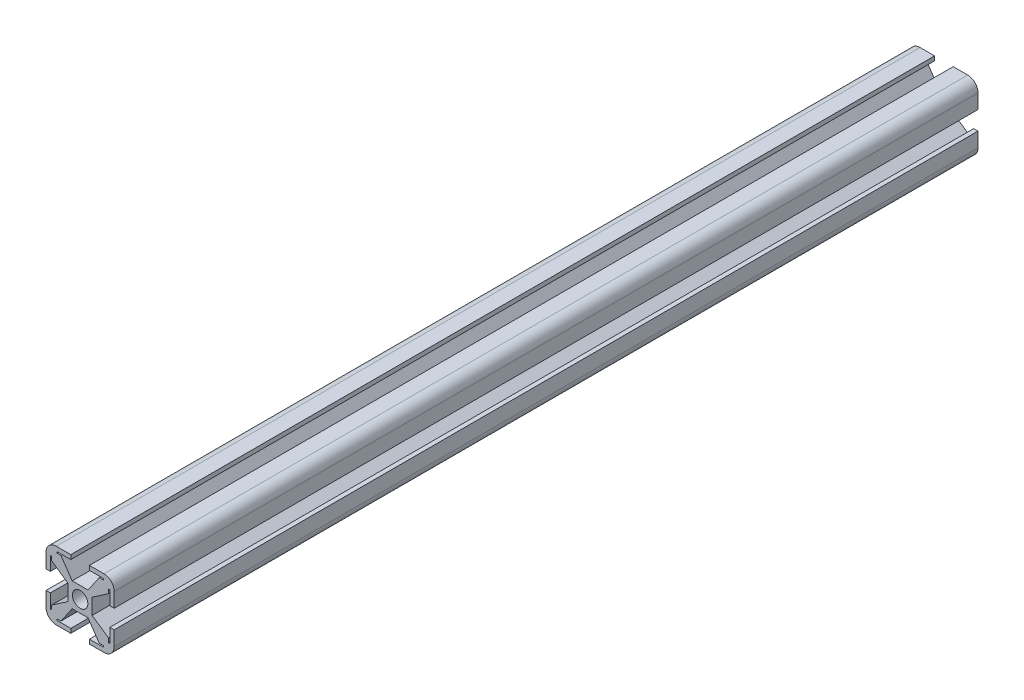
SolidWorks part; units mm, degrees
ref_plane "前视基准面" through (0, 0, 0) normal (0, 0, 1) x (1, 0, 0)
ref_plane "上视基准面" through (0, 0, 0) normal (0, 1, 0) x (1, 0, 0)
ref_plane "右视基准面" through (0, 0, 0) normal (1, 0, 0) x (0, 0, -1)
sketch "草图1" plane through (0, 0, 0) normal (0, 0, 1) x (1, 0, 0)
  line L1 (15, -15) -> (-15, -15)
  line L2 (15, -15) -> (15, 15)
  line L3 (15, 15) -> (-15, 15)
  line L4 (-15, -15) -> (-15, 15)
  line L5 (15, -15) -> (-15, 15) construction
  line L6 (15, 15) -> (-15, -15) construction
  point P0 (0, 0)
  dimension "D1" = 30
extrude "凸台-拉伸1" add sketch "草图1" along normal mid plane 380
fillet "圆角1" radius 4.5 4 edges at (15, -15, 0) (15, 15, 0) (-15, 15, 0) (-15, -15, 0)
sketch "草图2" plane through (0, 0, 190) normal (0, 0, 1) x (1, 0, 0)
  line L0 (10.5, 15) -> (-10.5, 15) construction
  line L1 (4.1, 17.2) -> (-4.1, 17.2)
  line L2 (4.1, 17.2) -> (4.1, 12.8)
  line L3 (4.1, 12.8) -> (-4.1, 12.8)
  line L4 (-4.1, 17.2) -> (-4.1, 12.8)
  line L5 (4.1, 17.2) -> (-4.1, 12.8) construction
  line L6 (4.1, 12.8) -> (-4.1, 17.2) construction
  line L7 (-10.25, 12.5) -> (-5.3, 5.3)
  line L8 (10.25, 13.1) -> (-10.25, 13.1)
  line L9 (10.25, 13.1) -> (10.25, 12.5)
  line L10 (10.25, 12.5) -> (-10.25, 12.5)
  line L11 (-10.25, 13.1) -> (-10.25, 12.5)
  line L12 (10.25, 13.1) -> (-10.25, 12.5) construction
  line L13 (10.25, 12.5) -> (-10.25, 13.1) construction
  line L14 (5.3, -5.3) -> (-5.3, -5.3)
  line L15 (5.3, -5.3) -> (5.3, 5.3)
  line L16 (5.3, 5.3) -> (-5.3, 5.3)
  line L17 (-5.3, -5.3) -> (-5.3, 5.3)
  line L18 (5.3, -5.3) -> (-5.3, 5.3) construction
  line L19 (5.3, 5.3) -> (-5.3, -5.3) construction
  line L20 (-8.4297, 12.5) -> (-3.4797, 5.3)
  line L21 (10.25, 12.5) -> (5.3, 5.3)
  line L22 (8.4297, 12.5) -> (3.4797, 5.3)
  circle A0 centre (0, 0) radius 3.4
  point P0 (0, 15)
  point P7 (0, 12.8)
  point P12 (0, 0)
  line M7 (10.5, 15) -> (-10.5, 15)
  dimension "D6" = 6.8
  dimension "D1" = 8.2
  dimension "D2" = 20.5
  dimension "D3" = 10.6
  dimension "D4" = 1.5
  dimension "D5" = 1.5
  dimension "D7" = 1.9
  dimension "D8" = 12.5
extrude "切除-拉伸1" cut sketch "草图2" against normal through all contours L2 L8 L4 L3 | L8 L2 L4 M7 | L8 L11 L10 L9 L2 L3 L4 | L22 L10 L20 L16 | A0
pattern_circular "阵列(圆周)1" count 4 over 360 about axis through (0, 0, 0) along (0, 0, 1) of "切除-拉伸1"
